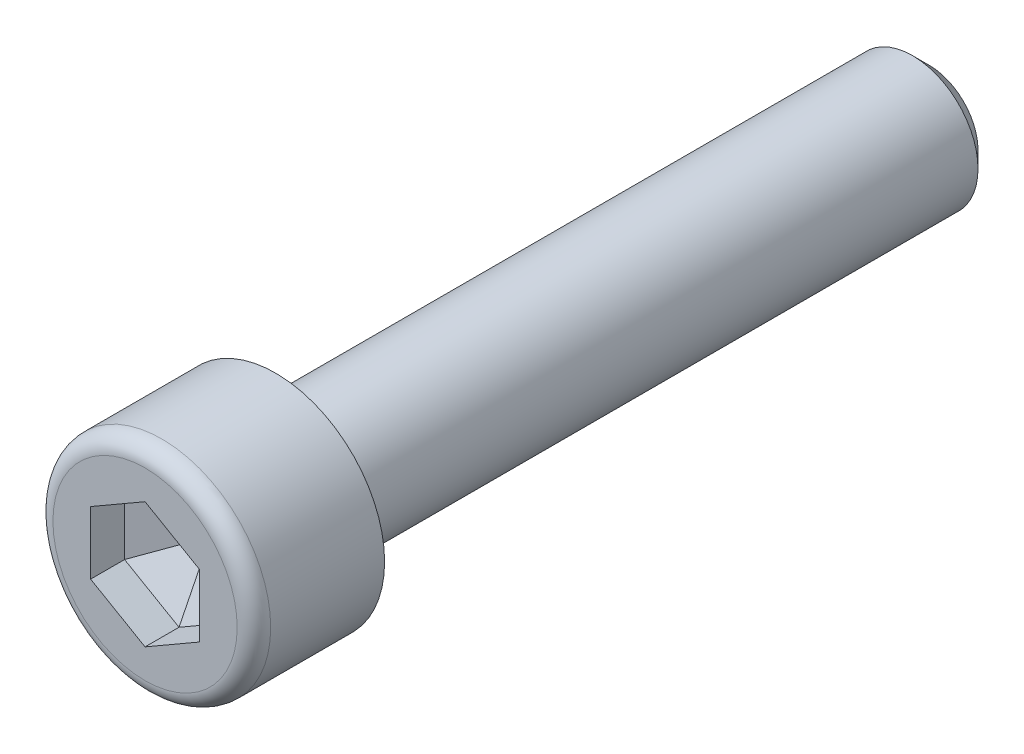
from build123d import *
from OCP.BRepFilletAPI import BRepFilletAPI_MakeChamfer

# Parameters (mm, degrees)
SKETCH1_R           = 5
BOSS_EXTRUDE1_DEPTH = 6
CUT_EXTRUDE1_DEPTH  = 3
SKETCH3_R           = 3
BOSS_EXTRUDE2_DEPTH = 30
CHAMFER1_SIZE       = 0.75
FILLET1_R           = 0.769230769
CHAMFER2_SIZE       = 1.44092219
CHAMFER2_SIZE2      = 2.495750443
FILLET2_R           = 0.1


with BuildPart() as part:
    # Sketch1 → Boss-Extrude1 (new body)
    with BuildSketch(Plane.XY):
        Circle(SKETCH1_R)
    extrude(amount=BOSS_EXTRUDE1_DEPTH)

    # Sketch2 → Cut-Extrude1 (cut)
    with BuildSketch(Plane.XY.offset(6)):
        Polygon((2.5, 1.443375673), (0, 2.886751346), (-2.5, 1.443375673), (-2.5, -1.443375673), (0, -2.886751346), (2.5, -1.443375673), align=None)
    extrude(amount=-CUT_EXTRUDE1_DEPTH, mode=Mode.SUBTRACT)

    # Sketch3 → Boss-Extrude2 (add)
    with BuildSketch(Plane(origin=(0, 0, 0), x_dir=(-1, 0, 0), z_dir=(0, 0, -1))):
        with Locations(Location((0, 0, 0), (0, 0, 180))):
            Circle(SKETCH3_R)
    extrude(amount=BOSS_EXTRUDE2_DEPTH)

    # Chamfer1
    chamfer1_edges = [part.edges().sort_by_distance(p)[0] for p in [
        (-3, 0, -30),
    ]]
    chamfer(chamfer1_edges, length=CHAMFER1_SIZE)

    # Fillet1
    fillet1_edges = [part.edges().sort_by_distance(p)[0] for p in [
        (-5, 0, 6),
    ]]
    fillet(fillet1_edges, radius=FILLET1_R)

    # Chamfer2: one chamfer whose edges measure the first distance from different faces: ONE call of the kernel's chamfer builder (chamfer() names one face for all edges)
    chamfer2_edges_1 = [part.edges().sort_by_distance(p)[0] for p in [
        (-1.25, 2.165063509, 3),
    ]]
    chamfer2_side_1 = [part.faces().sort_by_distance(p)[0] for p in [
        (-1.25, 2.165063509, 4.5),
    ]]
    chamfer2_edges_2 = [part.edges().sort_by_distance(p)[0] for p in [
        (1.25, 2.165063509, 3),
    ]]
    chamfer2_side_2 = [part.faces().sort_by_distance(p)[0] for p in [
        (1.25, 2.165063509, 4.5),
    ]]
    chamfer2_edges_3 = [part.edges().sort_by_distance(p)[0] for p in [
        (2.5, 0, 3),
    ]]
    chamfer2_side_3 = [part.faces().sort_by_distance(p)[0] for p in [
        (2.5, 0, 4.5),
    ]]
    chamfer2_edges_4 = [part.edges().sort_by_distance(p)[0] for p in [
        (1.25, -2.165063509, 3),
    ]]
    chamfer2_side_4 = [part.faces().sort_by_distance(p)[0] for p in [
        (1.25, -2.165063509, 4.5),
    ]]
    chamfer2_edges_5 = [part.edges().sort_by_distance(p)[0] for p in [
        (-1.25, -2.165063509, 3),
    ]]
    chamfer2_side_5 = [part.faces().sort_by_distance(p)[0] for p in [
        (-1.25, -2.165063509, 4.5),
    ]]
    chamfer2_edges_6 = [part.edges().sort_by_distance(p)[0] for p in [
        (-2.5, 0, 3),
    ]]
    chamfer2_side_6 = [part.faces().sort_by_distance(p)[0] for p in [
        (-2.5, 0, 4.5),
    ]]
    chamfer2 = BRepFilletAPI_MakeChamfer(part.part.solid().wrapped)
    for e in chamfer2_edges_1:
        chamfer2.Add(CHAMFER2_SIZE, CHAMFER2_SIZE2, e.wrapped, chamfer2_side_1[0].wrapped)  # the first distance lies on this face
    for e in chamfer2_edges_2:
        chamfer2.Add(CHAMFER2_SIZE, CHAMFER2_SIZE2, e.wrapped, chamfer2_side_2[0].wrapped)  # the first distance lies on this face
    for e in chamfer2_edges_3:
        chamfer2.Add(CHAMFER2_SIZE, CHAMFER2_SIZE2, e.wrapped, chamfer2_side_3[0].wrapped)  # the first distance lies on this face
    for e in chamfer2_edges_4:
        chamfer2.Add(CHAMFER2_SIZE, CHAMFER2_SIZE2, e.wrapped, chamfer2_side_4[0].wrapped)  # the first distance lies on this face
    for e in chamfer2_edges_5:
        chamfer2.Add(CHAMFER2_SIZE, CHAMFER2_SIZE2, e.wrapped, chamfer2_side_5[0].wrapped)  # the first distance lies on this face
    for e in chamfer2_edges_6:
        chamfer2.Add(CHAMFER2_SIZE, CHAMFER2_SIZE2, e.wrapped, chamfer2_side_6[0].wrapped)  # the first distance lies on this face
    add(Compound.cast(chamfer2.Shape()), mode=Mode.REPLACE)

    # Fillet2
    fillet2_edges = [part.edges().sort_by_distance(p)[0] for p in [
        (-3, 0, 0),
    ]]
    fillet(fillet2_edges, radius=FILLET2_R)


solid = part.part
